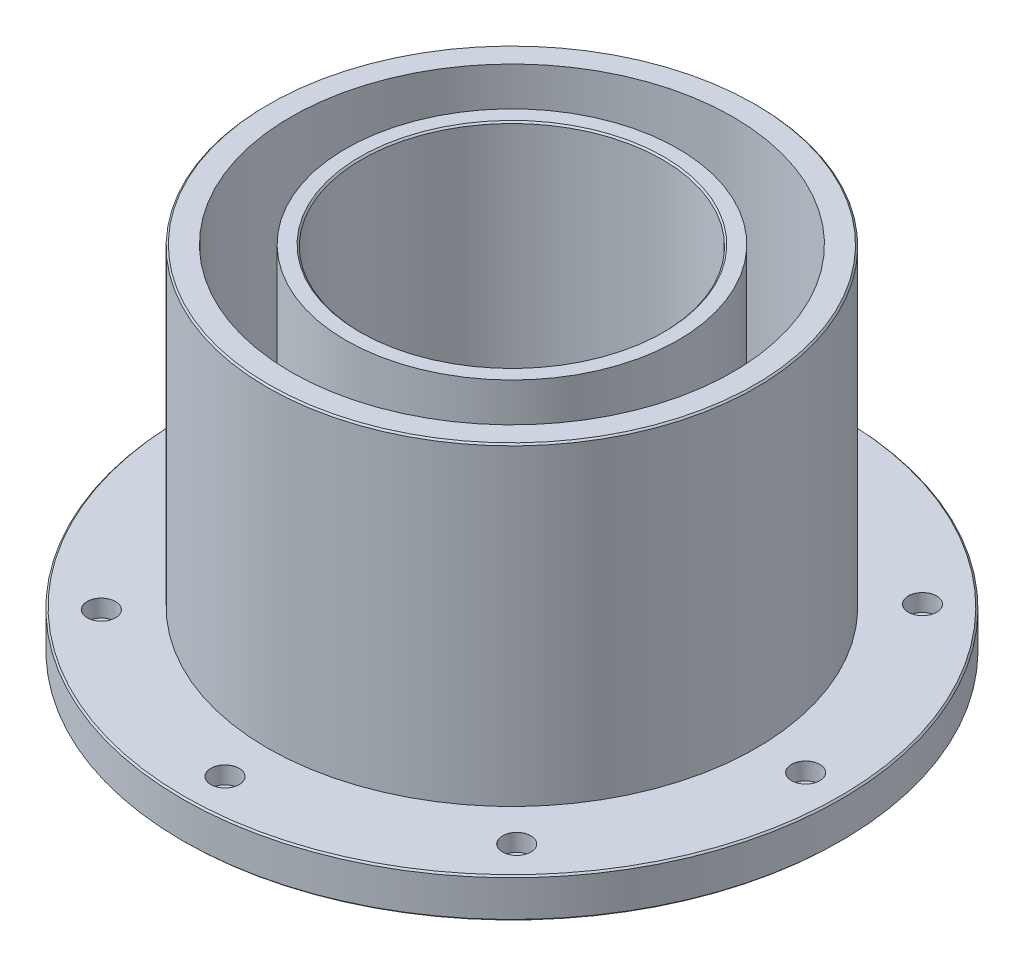
SolidWorks part; units mm, degrees
ref_plane "前视基准面" through (0, 0, 0) normal (0, 0, 1) x (1, 0, 0)
ref_plane "上视基准面" through (0, 0, 0) normal (0, 1, 0) x (1, 0, 0)
ref_plane "右视基准面" through (0, 0, 0) normal (1, 0, 0) x (0, 0, -1)
sketch "草图1" plane through (0, 0, 0) normal (0, 1, 0) x (1, 0, 0)
  circle A0 centre (0, 0) radius 210
  dimension "D1" = 420
extrude "凸台-拉伸1" add sketch "草图1" along normal blind 25 contours A0
sketch "草图2" plane through (0, 25, 0) normal (0, 1, 0) x (1, 0, 0)
  circle A0 centre (0, 0) radius 95.82
  circle A1 centre (0, 0) radius 100.82
  dimension "D1" = 191.64
  dimension "D2" = 201.64
extrude "切除-拉伸1" cut sketch "草图2" against normal blind 154 contours A0
sketch "草图3" plane through (0, 25, 0) normal (0, 1, 0) x (1, 0, 0)
  circle A0 centre (0, 0) radius 95.82
  circle A1 centre (0, 0) radius 155.82
  dimension "D1" = 191.64
  dimension "D2" = 311.64
extrude "凸台-拉伸2" add sketch "草图3" along normal blind 200 contours A1 | A0
chamfer "倒角1" distance 1 angle 45 4 edges at (0, 225, 95.82) (0, 225, 155.82) (0, 0, 210) (0, 25, 210)
sketch "草图7" plane through (0, 225, 0) normal (0, 1, 0) x (1, 0, 0)
  circle A0 centre (0, 0) radius 105.82
  circle A1 centre (0, 0) radius 140.82
  dimension "D1" = 211.64
  dimension "D2" = 281.64
extrude "切除-拉伸3" cut sketch "草图7" against normal blind 200 contours A1 | A0
sketch "草图8" plane through (0, 25, 0) normal (0, 1, 0) x (1, 0, 0)
  circle A0 centre (0, 0) radius 185 construction
  point P3 (-185, 0)
  dimension "D1" = 370
hole_wizard "M10 六角圆柱头螺钉的柱形沉头孔2" positions "草图9" profile "草图10" counterbore size "M10" standard "GB"
sketch "草图9" plane through (0, 25, 0) normal (0, 1, 0) x (1, 0, 0)
  circle A0 centre (0, 0) radius 185 construction
  point P0 (-184.9874, -2.159)
sketch "草图10" plane through (-184.9874, 25, 2.159) normal (1, 0, 0) x (0, 0, 1)
  line L0 (0, 0) -> (0, 30.8047)
  line L1 (0, 30.8047) -> (5.5, 27.5)
  line L2 (5.5, 27.5) -> (5.5, 11)
  line L3 (5.5, 11) -> (9, 11)
  line L5 (9, 11) -> (9, 0.025)
  line L6 (9, 0.025) -> (9.025, 0)
  line L7 (9.025, 0) -> (0, 0)
  line L8 (-9, 0.025) -> (-9.025, 0) construction
  line L10 (0, 30.8047) -> (-5.5, 27.5) construction
  line L11 (0, -6.35) -> (0, 107.95) construction
  dimension "孔直径" = 11
  dimension "孔深度" = 27.5
  dimension "锥形沉头孔直径" = 18
  dimension "锥形沉头孔深度" = 11
  dimension "近端锥形沉头孔直径" = 18.05
  dimension "近端锥形沉头孔角度" = 90
  dimension "导头角度" = 118
pattern_circular "阵列(圆周)2" count 8 every 45 about axis through (0, 0, 0) along (0, 1, 0) of "M10 六角圆柱头螺钉的柱形沉头孔2"
